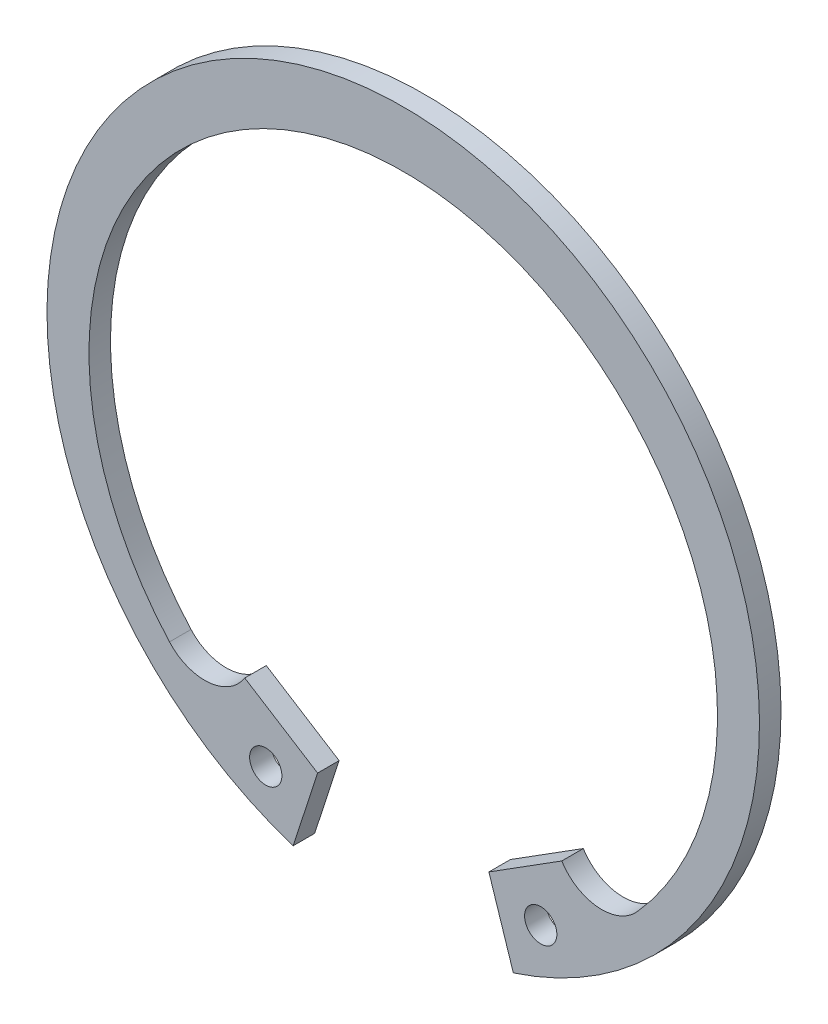
from build123d import *

# Parameters (mm, degrees)
BASE_EXTRUDE_DEPTH      = 1
BASE_EXTRUDE_DEPTH_BACK = 1
SKETCH1_R               = 1.5


with BuildPart() as part:
    # Sketch1 → Base-Extrude (new, two sides: drawn at the far end of the back side and taken through both)
    with BuildSketch(Plane.XY.offset(-BASE_EXTRUDE_DEPTH_BACK)):
        with BuildLine():
            Line((-14.724384167, -20.222967583), (-7.957187605, -24.489705295))
            Line((-7.957187605, -24.489705295), (-10.228462514, -31.479970689))
            ThreePointArc((-10.228462514, -31.479970689), (0, 33.1), (10.228462514, -31.479970689))
            Line((10.228462514, -31.479970689), (7.957187605, -24.489705295))
            Line((7.957187605, -24.489705295), (14.724384167, -20.222967583))
            ThreePointArc((14.724384167, -20.222967583), (18.073876023, -22.260468599), (21.719080421, -20.817211524))
            ThreePointArc((21.719080421, -20.817211524), (0, 27.9), (-21.719080421, -20.817211524))
            ThreePointArc((-21.719080421, -20.817211524), (-18.073876023, -22.260468599), (-14.724384167, -20.222967583))
        make_face()
        with Locations((-12.773653929, -26.368992497)):
            Circle(SKETCH1_R, mode=Mode.SUBTRACT)
        with Locations(Location((12.773653929, -26.368992497, 0), (0, 0, 180))):
            Circle(SKETCH1_R, mode=Mode.SUBTRACT)
    extrude(amount=BASE_EXTRUDE_DEPTH + BASE_EXTRUDE_DEPTH_BACK)


solid = part.part
